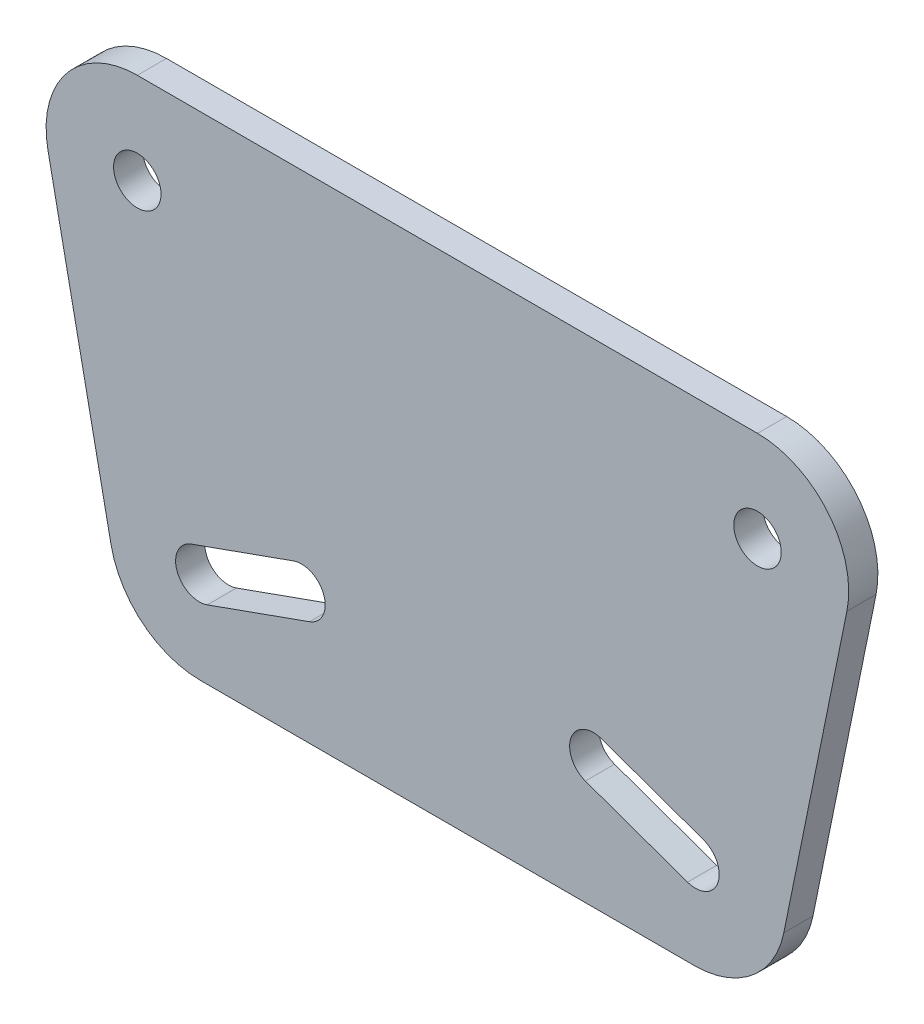
from build123d import *

# Parameters (mm, degrees)
SKETCH1_R           = 6.5
BOSS_EXTRUDE1_DEPTH = 8


with BuildPart() as part:
    # Sketch1 → Boss-Extrude1 (new body)
    with BuildSketch(Plane.XY):
        with BuildLine():
            Line((0, 0), (170, 0))
            ThreePointArc((170, 0), (189.359816102, -9.182366786), (194.498117616, -29.98419836))
            Line((194.498117616, -29.98419836), (177.204672165, -114.98419836))
            ThreePointArc((177.204672165, -114.98419836), (168.524187763, -129.359816102), (152.706554549, -135))
            Line((152.706554549, -135), (17.293445451, -135))
            ThreePointArc((17.293445451, -135), (1.475812237, -129.359816102), (-7.204672165, -114.98419836))
            Line((-7.204672165, -114.98419836), (-24.498117616, -29.98419836))
            ThreePointArc((-24.498117616, -29.98419836), (-19.359816102, -9.182366786), (0, 0))
        make_face()
        with Locations((0, -25)):
            Circle(SKETCH1_R, mode=Mode.SUBTRACT)
        with Locations((170, -25)):
            Circle(SKETCH1_R, mode=Mode.SUBTRACT)
        with BuildLine():
            Line((14.81381342, -103.878677575), (42.81381342, -93.878677575))
            ThreePointArc((42.81381342, -93.878677575), (51.121322425, -97.81381342), (47.18618658, -106.121322425))
            Line((47.18618658, -106.121322425), (19.18618658, -116.121322425))
            ThreePointArc((19.18618658, -116.121322425), (10.878677575, -112.18618658), (14.81381342, -103.878677575))
        make_face(mode=Mode.SUBTRACT)
        with BuildLine():
            Line((127.18618658, -93.878677575), (155.18618658, -103.878677575))
            ThreePointArc((155.18618658, -103.878677575), (159.121322425, -112.18618658), (150.81381342, -116.121322425))
            Line((150.81381342, -116.121322425), (122.81381342, -106.121322425))
            ThreePointArc((122.81381342, -106.121322425), (118.878677575, -97.81381342), (127.18618658, -93.878677575))
        make_face(mode=Mode.SUBTRACT)
    extrude(amount=BOSS_EXTRUDE1_DEPTH)


solid = part.part
